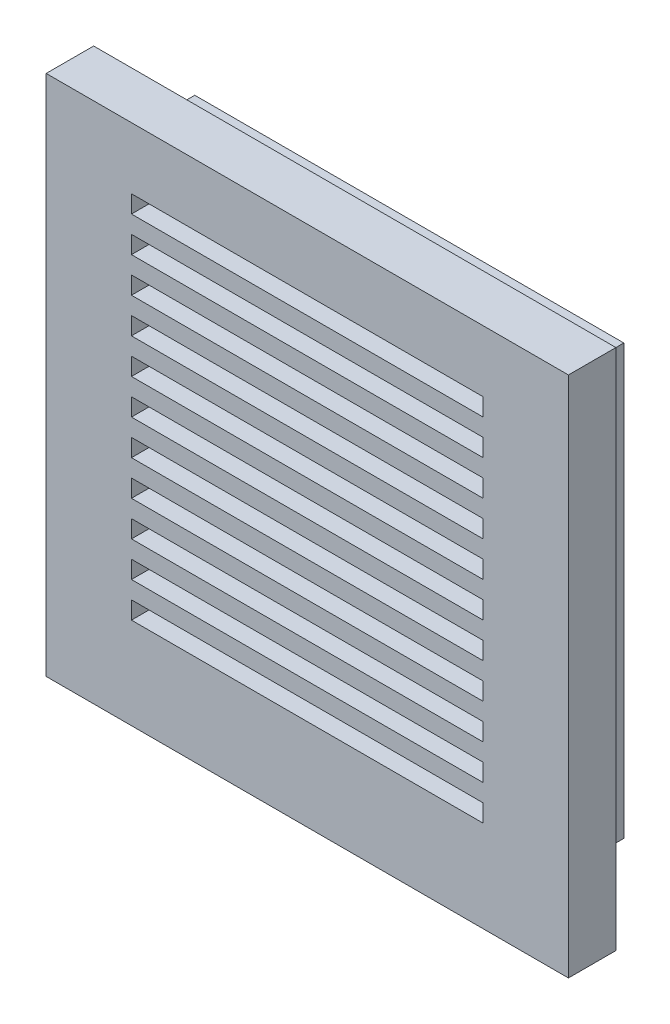
from build123d import *

# Parameters (mm, degrees)
SKETCH_1_W             = 122
SKETCH_1_H             = 122
EXTRUDE_1_DEPTH        = 15.5
SKETCH_2_W             = 148.5
SKETCH_2_H             = 148.5
EXTRUDE_2_DEPTH        = 13.5
SKETCH_3_W             = 100
SKETCH_3_H             = 5
CUT_EXTRUDE_1_DEPTH    = 109.936334618
PATTERN_LINEAR_1_COUNT = 11
PATTERN_LINEAR_1_PITCH = 10
MM_1_D                 = 5
MM_1_DEPTH             = 10
MM_1_TIP               = 1.502151548
HOLE_WIZARD_M4_1_D     = 3.3
HOLE_WIZARD_M4_1_DEPTH = 10.1
HOLE_WIZARD_M4_1_TIP   = 0.991420021


with BuildPart() as part:
    # 草图1 → 凸台-拉伸1 (new body)
    with BuildSketch(Plane.XY):
        Rectangle(SKETCH_1_W, SKETCH_1_H)
    extrude(amount=EXTRUDE_1_DEPTH)

    # 草图2 → 凸台-拉伸2 (add)
    with BuildSketch(Plane.XY.offset(15.5)):
        Rectangle(SKETCH_2_W, SKETCH_2_H)
    extrude(amount=EXTRUDE_2_DEPTH)

    # 草图3 → 切除-拉伸1 (cut, through all)
    with BuildSketch(Plane.XY.offset(29)):
        with Locations((0, 54.25)):
            Rectangle(SKETCH_3_W, SKETCH_3_H)
    cut_extrude_1 = extrude(amount=-CUT_EXTRUDE_1_DEPTH, mode=Mode.SUBTRACT)

    # 阵列(线性)1: 切除-拉伸1 ×11
    with Locations(*[(0, -i * PATTERN_LINEAR_1_PITCH, 0) for i in range(1, PATTERN_LINEAR_1_COUNT)]):
        add(cut_extrude_1, mode=Mode.SUBTRACT)

    # 大小mm 暗销孔1
    with Locations(Plane(origin=(0, 0, 15.5), x_dir=(-1, 0, 0), z_dir=(0, 0, -1))):
        with Locations((-65.5, 65.5), (0, 65.5), (65.5, 65.5), (65.5, 0), (-65.5, 0), (-65.5, -65.5), (0, -65.5), (65.5, -65.5)):
            Hole(MM_1_D / 2, depth=MM_1_DEPTH)
            with Locations((0, 0, -(MM_1_DEPTH + MM_1_TIP / 2))):  # 118° drill point
                Cone(0, MM_1_D / 2, MM_1_TIP, mode=Mode.SUBTRACT)

    # M4 螺纹孔1
    with Locations(Plane(origin=(0, 0, 0), x_dir=(-1, 0, 0), z_dir=(0, 0, -1))):
        with Locations((-52.5, 52.5), (52.5, 52.5), (52.5, -52.5), (-52.5, -52.5)):
            Hole(HOLE_WIZARD_M4_1_D / 2, depth=HOLE_WIZARD_M4_1_DEPTH)
            with Locations((0, 0, -(HOLE_WIZARD_M4_1_DEPTH + HOLE_WIZARD_M4_1_TIP / 2))):  # 118° drill point
                Cone(0, HOLE_WIZARD_M4_1_D / 2, HOLE_WIZARD_M4_1_TIP, mode=Mode.SUBTRACT)


solid = part.part
